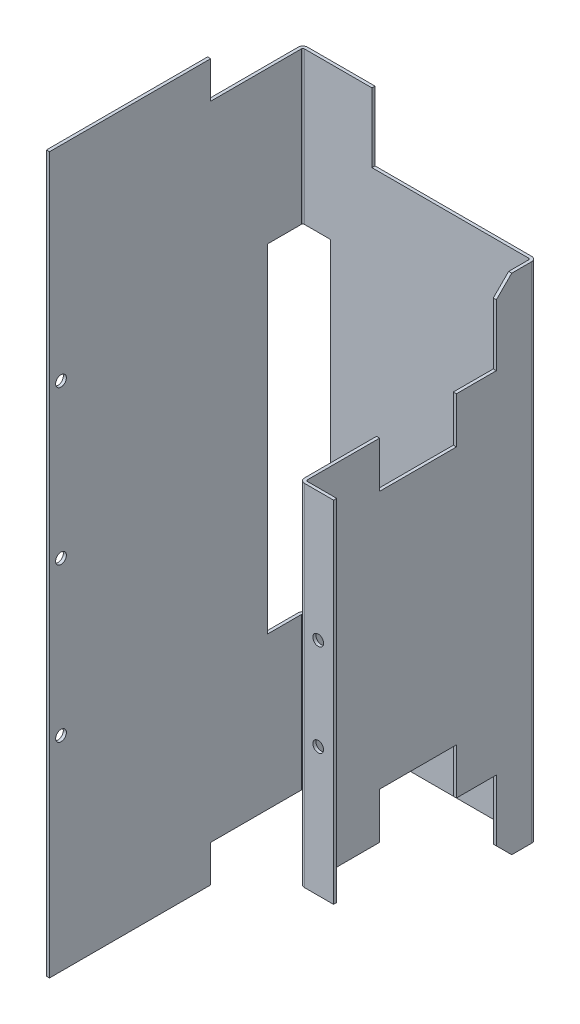
SolidWorks part; units mm, degrees
ref_plane "Front Plane" through (0, 0, 0) normal (0, 0, 1) x (1, 0, 0)
ref_plane "Top Plane" through (0, 0, 0) normal (0, 1, 0) x (1, 0, 0)
ref_plane "Right Plane" through (0, 0, 0) normal (1, 0, 0) x (0, 0, -1)
sketch "Sketch1" plane through (0, 0, 0) normal (0, 1, 0) x (1, 0, 0)
  line L0 (0, 0) -> (0, 165)
  line L1 (0, 165) -> (148, 165)
  line L2 (148, 165) -> (148, 15)
  line L3 (148, 15) -> (170, 15)
  line L4 (-2, 0) -> (-2, 167)
  line L5 (-2, 167) -> (150, 167)
  line L6 (150, 167) -> (150, 17)
  line L7 (150, 17) -> (170, 17)
  line L8 (-2, 0) -> (0, 0)
  line L9 (170, 17) -> (170, 15)
  dimension "D1" = 165
  dimension "D2" = 148
  dimension "D3" = 22
  dimension "D4" = 150
  dimension "D5" = 2
extrude "Boss-Extrude1" add sketch "Sketch1" along normal blind 418
sketch "Sketch2" plane through (0, 0, -167) normal (0, 0, -1) x (-1, 0, 0)
  line L0 (2, 418) -> (2, 0) construction
  line L1 (2, 99) -> (-18, 99)
  line L2 (2, 99) -> (2, 319)
  line L3 (2, 319) -> (-18, 319)
  line L4 (-18, 99) -> (-18, 319)
  line L5 (-150, 418) -> (-150, 0) construction
  point P6 (-150, 209)
  dimension "D1" = 220
  dimension "D2" = 110
  dimension "D3" = 20
extrude "Cut-Extrude1" cut sketch "Sketch2" against normal blind 25
sketch "Sketch3" plane through (0, 0, -167) normal (0, 0, -1) x (-1, 0, 0)
  line L1 (-170, 418) -> (-45, 418)
  line L2 (-170, 418) -> (-170, 373)
  line L3 (-170, 373) -> (-45, 373)
  line L4 (-45, 418) -> (-45, 373)
  line L5 (-170, 0) -> (-45, 0)
  line L6 (-170, 0) -> (-170, 45)
  line L7 (-170, 45) -> (-45, 45)
  line L8 (-45, 0) -> (-45, 45)
  dimension "D1" = 45
  dimension "D2" = 45
  dimension "D3" = 125
  dimension "D4" = 125
extrude "Cut-Extrude2" cut sketch "Sketch3" against normal through all
fillet "Fillet1" radius 3 4 edges at (148, 209, -15) (150, 209, -167) (-2, 49.5, -167) (-2, 368.5, -167)
fillet "Fillet2" radius 1 4 edges at (0, 368.5, -165) (0, 49.5, -165) (148, 209, -165) (150, 209, -17)
sketch "Sketch5" plane through (0, 0, -17) normal (0, 0, -1) x (-1, 0, 0)
  line L0 (-170, 373) -> (-170, 45) construction
  circle A0 centre (-160, 239) radius 3.5
  circle A1 centre (-160, 179) radius 3.5
  point P4 (-170, 209)
  point P7 (-170, 209)
  dimension "D3" = 7
  dimension "D6" = 7
  dimension "D1" = 30
  dimension "D2" = 10
  dimension "D4" = 30
  dimension "D5" = 10
extrude "Cut-Extrude4" cut sketch "Sketch5" against normal through all
sketch "Sketch6" plane through (-2, 0, 0) normal (-1, 0, 0) x (0, 0, 1)
  line L0 (0, 418) -> (0, 0) construction
  circle A0 centre (-7.5, 309) radius 3.5
  circle A1 centre (-7.5, 209) radius 3.5
  circle A2 centre (-7.5, 109) radius 3.5
  point P8 (0, 209)
  point P9 (0, 209)
  point P10 (0, 209)
  dimension "D2" = 7
  dimension "D1" = 7.5
  dimension "D3" = 100
  dimension "D4" = 100
  dimension "D5" = 0
extrude "Cut-Extrude5" cut sketch "Sketch6" against normal up to next
sketch "Sketch8" plane through (0, 0, 0) normal (0, -1, 0) x (1, 0, 0)
  line L0 (0, 0) -> (0, -164) construction
  line L1 (-2, 0) -> (0, 0)
  line L2 (-2, 0) -> (-2, -105)
  line L3 (-2, -105) -> (0, -105)
  line L4 (0, 0) -> (0, -105)
  dimension "D1" = 105
extrude "Boss-Extrude2" add sketch "Sketch8" along normal blind 24
sketch "Sketch9" plane through (0, 418, 0) normal (0, 1, 0) x (1, 0, 0)
  line L0 (0, 0) -> (0, 164) construction
  line L1 (-2, 0) -> (0, 0)
  line L2 (-2, 0) -> (-2, 105)
  line L3 (-2, 105) -> (0, 105)
  line L4 (0, 0) -> (0, 105)
  dimension "D1" = 105
extrude "Boss-Extrude3" add sketch "Sketch9" along normal blind 24
sketch "Sketch10" plane through (150, 0, 0) normal (1, 0, 0) x (0, 0, -1)
  line L0 (24.7685, 209) -> (164, 209) construction
  line L1 (15, 373) -> (141, 373)
  line L2 (15, 373) -> (15, 323)
  line L3 (15, 323) -> (141, 323)
  line L4 (141, 373) -> (141, 323)
  line L5 (164, 45) -> (164, 373) construction
  line L6 (141, 45) -> (141, 95)
  line L7 (15, 45) -> (141, 45)
  line L8 (15, 45) -> (15, 95)
  line L9 (15, 95) -> (141, 95)
  line L10 (164, 373) -> (18, 373) construction
  line L11 (15, 373) -> (15, 45) construction
  dimension "D1" = 50
  dimension "D2" = 126
extrude "Cut-Extrude6" cut sketch "Sketch10" against normal blind 10 and the other way blind 30
chamfer "Chamfer1" distance 10 angle 45 2 edges at (149, 373, -141) (149, 45, -141)
sketch "Sketch11" plane through (150, 0, 0) normal (1, 0, 0) x (0, 0, -1)
  line L0 (141, 95) -> (18, 95) construction
  line L1 (65, 95) -> (115, 95)
  line L2 (65, 95) -> (65, 125)
  line L3 (65, 125) -> (115, 125)
  line L4 (115, 95) -> (115, 125)
  line L5 (15, 323) -> (15, 95) construction
  line L6 (15, 209) -> (148.0396, 209) construction
  line L7 (65, 323) -> (115, 323)
  line L8 (65, 323) -> (65, 293)
  line L9 (65, 293) -> (115, 293)
  line L10 (115, 323) -> (115, 293)
  dimension "D1" = 30
  dimension "D2" = 50
  dimension "D3" = 50
extrude "Cut-Extrude7" cut sketch "Sketch11" against normal blind 10
